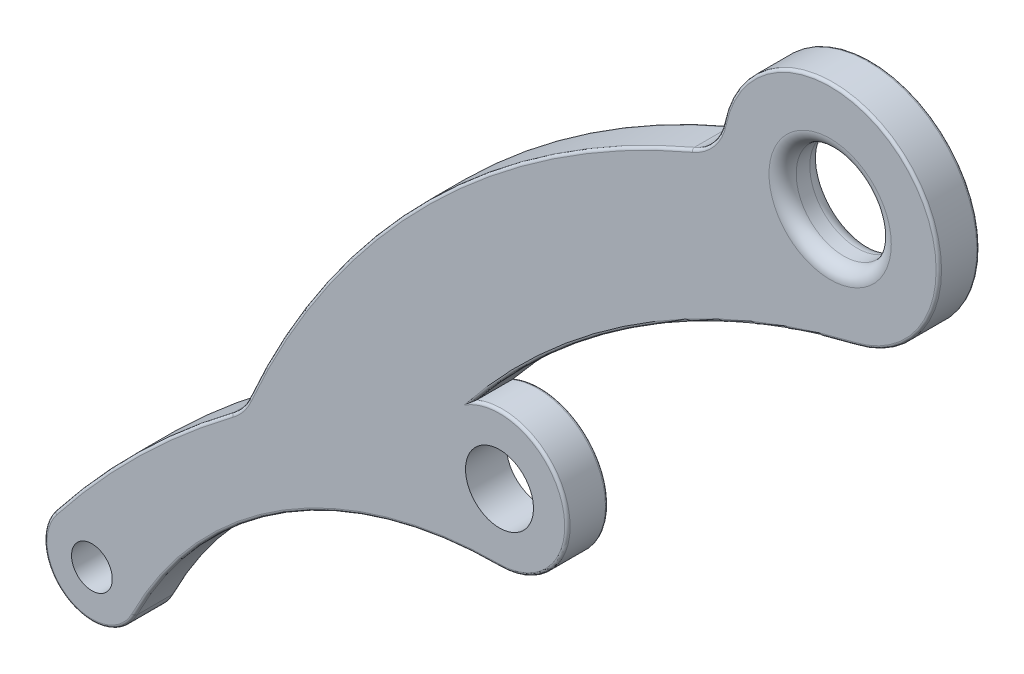
from build123d import *

# Parameters (mm, degrees)
BOSS_EXTRUDE1_DEPTH        = 15
M30_CLEARANCE_HOLE1_D      = 35
F_25_0_25_DIAMETER_HOLE1_D = 25
F_15_0_15_DIAMETER_HOLE1_D = 15
FILLET1_R                  = 20
FILLET2_R                  = 1
FILLET3_R                  = 5


with BuildPart() as part:
    # Sketch1 → Boss-Extrude1 (new body)
    with BuildSketch(Plane.XY.offset(15)):
        with BuildLine():
            ThreePointArc((231.736862835, 248.122711482), (126.150277633, 181.071444034), (55.655412109, 77.752165214))
            ThreePointArc((55.655412109, 77.752165214), (18.626786765, 46.68025613), (-13.767622093, 10.802896922))
            ThreePointArc((-13.767622093, 10.802896922), (-9.366641165, -14.782287823), (15.647688545, -7.835805205))
            ThreePointArc((15.647688545, -7.835805205), (71.03368715, 52.673473852), (149.967247602, 75.000021454))
            ThreePointArc((149.967247602, 75.000021454), (174.552001265, 104.711606298), (140.715233091, 123.211917272))
            ThreePointArc((140.715233091, 123.211917272), (203.688662251, 178.625691043), (281.028515533, 211.104702698))
            ThreePointArc((281.028515533, 211.104702698), (295.713241867, 281.984647802), (231.736862835, 248.122711482))
        make_face()
    extrude(amount=-BOSS_EXTRUDE1_DEPTH)

    # M30 Clearance Hole1 (through all)
    with Locations(Plane(origin=(0, 0, 0), x_dir=(-1, 0, 0), z_dir=(0, 0, -1))):
        with Locations((-271.692785898, 250)):
            Hole(M30_CLEARANCE_HOLE1_D / 2)

    # Ø25.0 (25) Diameter Hole1 (through all)
    with Locations(Plane(origin=(0, 0, 0), x_dir=(-1, 0, 0), z_dir=(0, 0, -1))):
        with Locations((-150, 100)):
            Hole(F_25_0_25_DIAMETER_HOLE1_D / 2)

    # Ø15.0 (15) Diameter Hole1 (through all)
    with Locations(Plane(origin=(0, 0, 0), x_dir=(-1, 0, 0), z_dir=(0, 0, -1))):
        with Locations((0, 0)):
            Hole(F_15_0_15_DIAMETER_HOLE1_D / 2)

    # Fillet1
    fillet1_edges = [part.edges().sort_by_distance(p)[0] for p in [
        (55.655412109, 77.752165214, 7.5),
        (231.736862835, 248.122711482, 7.5),
    ]]
    fillet(fillet1_edges, radius=FILLET1_R)

    # Fillet2
    fillet2_edges = [part.edges().sort_by_distance(p)[0] for p in [
        (299.518468185, 278.735542543, 15),
        (-9.366641165, -14.782287823, 0),
        (71.03368715, 52.673473852, 0),
        (174.552001265, 104.711606298, 0),
        (203.688662251, 178.625691043, 0),
        (123.791931468, 178.765167219, 15),
        (123.791931468, 178.765167219, 0),
        (16.734224094, 44.841311513, 15),
        (16.734224094, 44.841311513, 0),
        (228.397133093, 249.440841249, 15),
        (228.397133093, 249.440841249, 0),
        (55.082608051, 78.193527318, 15),
        (55.082608051, 78.193527318, 0),
        (299.518468185, 278.735542543, 0),
        (203.688662251, 178.625691043, 15),
        (174.552001265, 104.711606298, 15),
        (71.03368715, 52.673473852, 15),
        (-9.366641165, -14.782287823, 15),
    ]]
    fillet(fillet2_edges, radius=FILLET2_R)

    # Fillet3
    fillet3_edges = [part.edges().sort_by_distance(p)[0] for p in [
        (254.192785898, 250, 0),
        (254.192785898, 250, 15),
    ]]
    fillet(fillet3_edges, radius=FILLET3_R)


solid = part.part
